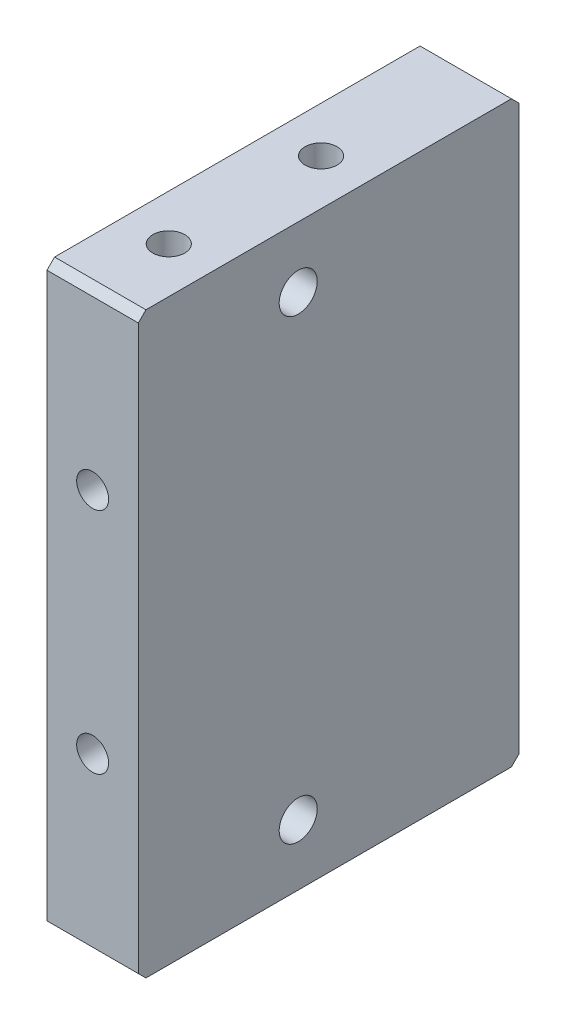
SolidWorks part; units mm, degrees
material "A7075"
ref_plane "Front Plane" through (0, 0, 0) normal (0, 0, 1) x (1, 0, 0)
ref_plane "Top Plane" through (0, 0, 0) normal (0, 1, 0) x (1, 0, 0)
ref_plane "Right Plane" through (0, 0, 0) normal (1, 0, 0) x (0, 0, -1)
sketch "Sketch6" plane through (0, 0, 0) normal (1, 0, 0) x (0, 0, -1)
  line L1 (0, 38) -> (50, 38)
  line L2 (0, 38) -> (0, -38)
  line L3 (0, -38) -> (50, -38)
  line L4 (50, 38) -> (50, -38)
  dimension "D1" = 76
  dimension "D2" = 50
extrude "Boss-Extrude6" add sketch "Sketch6" against normal blind 12 separate body
hole_wizard "M6 Tapped Hole2" positions "Sketch18" profile "Sketch17" tap size "M6" standard "Iso"
sketch "Sketch18" plane through (0, 0, 0) normal (1, 0, 0) x (0, 0, -1)
  line L1 (0, 38) -> (0, -38) construction
  point P0 (21, -30)
  point P2 (21, 30)
  dimension "D1" = 60
  dimension "D2" = 30
  dimension "D3" = 21
sketch "Sketch17" plane through (0, -30, -21) normal (0, 1, 0) x (0, 0, -1)
  line L0 (0, 0) -> (0, 16.5022)
  line L1 (0, 16.5022) -> (2.5, 15)
  line L2 (2.5, 15) -> (2.5, 0)
  line L5 (2.5, 0) -> (0, 0)
  line L10 (0, 16.5022) -> (-2.5, 15) construction
  line L11 (0, -6.35) -> (0, 107.95) construction
  dimension "螺纹孔钻头直径" = 5
  dimension "螺纹孔钻头深度" = 15
  dimension "导头角度" = 118
cosmetic thread "Cosmetic thread 10" parameters "D1"=12, "D2"=6
cosmetic thread "Cosmetic thread 11" parameters "D1"=12, "D2"=6
hole_wizard "M5 Tapped Hole3" positions "Sketch20" profile "Sketch19" tap size "M5" standard "Iso"
sketch "Sketch20" plane through (0, -38, 0) normal (0, -1, 0) x (-1, 0, 0)
  line L0 (12, 0) -> (0, 0) construction
  point P0 (6, 10)
  point P2 (6, 30)
  point P7 (6, 0)
  dimension "D1" = 10
  dimension "D2" = 20
sketch "Sketch19" plane through (-6, -38, -10) normal (1, 0, 0) x (0, 0, -1)
  line L0 (0, 0) -> (0, 18.6618)
  line L1 (0, 18.6618) -> (2.1, 17.4)
  line L2 (2.1, 17.4) -> (2.1, 0)
  line L5 (2.1, 0) -> (0, 0)
  line L10 (0, 18.6618) -> (-2.1, 17.4) construction
  line L11 (0, -6.35) -> (0, 107.95) construction
  dimension "螺纹孔钻头直径" = 4.2
  dimension "螺纹孔钻头深度" = 17.4
  dimension "导头角度" = 118
cosmetic thread "Cosmetic thread 25" parameters "D1"=15, "D2"=5
cosmetic thread "Cosmetic thread 26" parameters "D1"=15, "D2"=5
mirror "Mirror1" about plane through (0, 0, 0) normal (0, 1, 0) of "M5 Tapped Hole3"
hole_wizard "M5 Tapped Hole2" positions "Sketch22" profile "Sketch21" tap size "M5" standard "Iso"
sketch "Sketch22" plane through (0, 0, 0) normal (0, 0, 1) x (1, 0, 0)
  line L0 (-12, 38) -> (-12, -38) construction
  point P0 (-6, 15)
  point P2 (-6, -15)
  dimension "D1" = 30
  dimension "D2" = 15
  dimension "D3" = 6
sketch "Sketch21" plane through (-6, 15, 0) normal (1, 0, 0) x (0, -1, 0)
  line L0 (0, 0) -> (0, 13.6618)
  line L1 (0, 13.6618) -> (2.1, 12.4)
  line L2 (2.1, 12.4) -> (2.1, 0)
  line L5 (2.1, 0) -> (0, 0)
  line L10 (0, 13.6618) -> (-2.1, 12.4) construction
  line L11 (0, -6.35) -> (0, 107.95) construction
  dimension "螺纹孔钻头直径" = 4.2
  dimension "螺纹孔钻头深度" = 12.4
  dimension "导头角度" = 118
cosmetic thread "Cosmetic thread 27" parameters "D1"=10, "D2"=5
cosmetic thread "Cosmetic thread 28" parameters "D1"=10, "D2"=5
chamfer "Chamfer1" distance 1 angle 45 4 edges at (-6, 38, 0) (-6, 38, -50) (-6, -38, -50) (-6, -38, 0)
